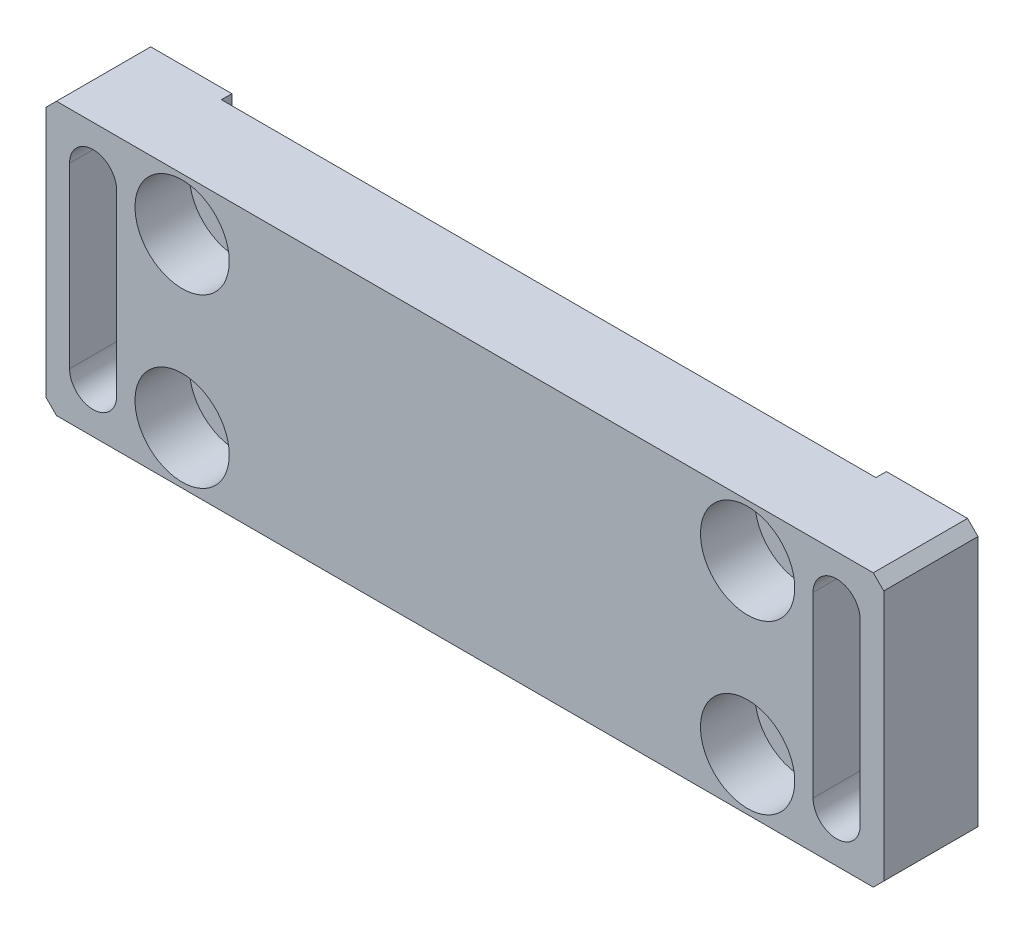
SolidWorks part; units mm, degrees
material "A6063"
ref_plane "Front Plane" through (0, 0, 0) normal (0, 0, 1) x (1, 0, 0)
ref_plane "Top Plane" through (0, 0, 0) normal (0, 1, 0) x (1, 0, 0)
ref_plane "Right Plane" through (0, 0, 0) normal (1, 0, 0) x (0, 0, -1)
sketch "Sketch1" plane through (0, 0, 0) normal (0, 0, 1) x (1, 0, 0)
  line L1 (-40, 13) -> (40, 13)
  line L2 (-40, 13) -> (-40, -13)
  line L3 (-40, -13) -> (40, -13)
  line L4 (40, 13) -> (40, -13)
  line L5 (-40, 13) -> (40, -13) construction
  line L6 (-40, -13) -> (40, 13) construction
  point P0 (0, 0)
  dimension "D1" = 80
  dimension "D2" = 26
extrude "Boss-Extrude1" add sketch "Sketch1" along normal blind 9
sketch "Sketch2" plane through (0, 0, 9) normal (0, 0, 1) x (1, 0, 0)
  line L0 (-40, 13) -> (-40, -13) construction
  line L1 (-40, 0) -> (41.3444, 0) construction
  line L3 (0, 0) -> (0, -13) construction
  line L4 (-40, -13) -> (40, -13) construction
  circle A8 centre (-27, -8) radius 2.6
  circle A9 centre (-27, 8) radius 2.6
  circle A10 centre (27, 8) radius 2.6
  circle A11 centre (27, -8) radius 2.6
  dimension "D1" = 5.2
  dimension "D2" = 16
  dimension "D4" = 54
  dimension "D5" = 13
extrude "Cut-Extrude1" cut sketch "Sketch2" against normal up to next
sketch "Sketch3" plane through (0, 0, 9) normal (0, 0, 1) x (1, 0, 0)
  circle A0 centre (-27, -8) radius 4.5
  circle A1 centre (-27, 8) radius 4.5
  circle A2 centre (27, 8) radius 4.5
  circle A3 centre (27, -8) radius 4.5
  dimension "D1" = 9
extrude "Cut-Extrude2" cut sketch "Sketch3" against normal blind 5.2
sketch "Sketch6" plane through (0, 0, 0) normal (0, 0, -1) x (-1, 0, 0)
  line L0 (-35.5, 8.5) -> (-35.5, -8.5) construction
  line L1 (-33.25, 8.5) -> (-33.25, -8.5)
  line L2 (-37.75, 8.5) -> (-37.75, -8.5)
  line L3 (-40, 0) -> (43.6983, 0) construction
  line L4 (-40, -13) -> (-40, 13) construction
  arc A0 (-33.25, 8.5) -> (-37.75, 8.5) centre (-35.5, 8.5) ccw
  arc A1 (-37.75, -8.5) -> (-33.25, -8.5) centre (-35.5, -8.5) ccw
  point P3 (-35.5, 0)
  dimension "D3" = 2.25
  dimension "D1" = 17
  dimension "D2" = 4.5
extrude "Cut-Extrude3" cut sketch "Sketch6" against normal up to next
mirror "Mirror1" about plane through (0, 0, 0) normal (1, 0, 0) of "Cut-Extrude3"
sketch "Sketch8" plane through (0, 0, 0) normal (0, 0, -1) x (-1, 0, 0)
  line L0 (40, -13) -> (-40, -13) construction
  line L1 (-31.25, 13) -> (31.25, 13)
  line L2 (-31.25, 13) -> (-31.25, -13)
  line L3 (-31.25, -13) -> (31.25, -13)
  line L4 (31.25, 13) -> (31.25, -13)
  line L5 (-31.25, 13) -> (31.25, -13) construction
  line L6 (-31.25, -13) -> (31.25, 13) construction
  point P0 (0, 0)
  dimension "D1" = 62.5
extrude "Cut-Extrude5" cut sketch "Sketch8" against normal blind 1
chamfer "Chamfer1" distance 1 angle 45 4 edges at (40, 13, 4.5) (40, -13, 4.5) (-40, -13, 4.5) (-40, 13, 4.5)
